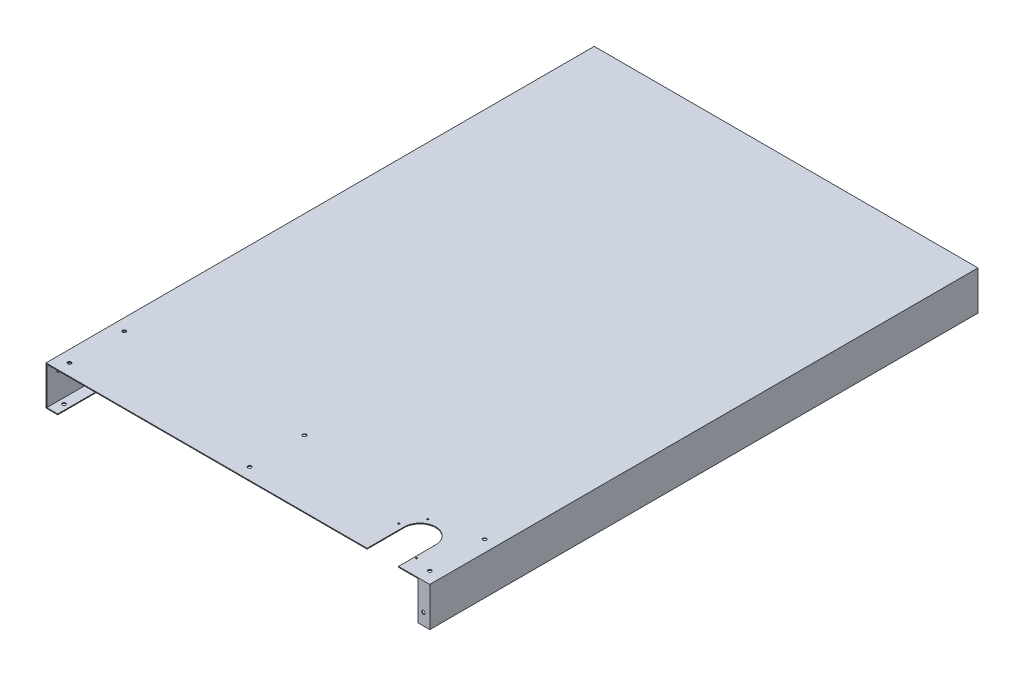
from build123d import *

# Parameters (mm, degrees)
SKETCH_1_W             = 980
SKETCH_1_H             = 1400
EXTRUDE_1_DEPTH        = 100
SHELL_1_T              = -2
CUT_EXTRUDE_1_DEPTH    = 20
SKETCH_5_W             = 976
SKETCH_5_H             = 98
CUT_EXTRUDE_2_DEPTH    = 20
EXTRUDE_2_DEPTH        = 2
SKETCH_7_W             = 2
SKETCH_7_H             = 96
EXTRUDE_3_DEPTH        = 28
SKETCH_8_R             = 4.5
CUT_EXTRUDE_3_DEPTH    = 10
SKETCH_9_R             = 4.5
CUT_EXTRUDE_4_DEPTH    = 10
SKETCH_10_R            = 4.5
CUT_EXTRUDE_5_DEPTH    = 10
SKETCH_11_R            = 4.5
CUT_EXTRUDE_6_DEPTH    = 10
HOLE_WIZARD_M5_1_D     = 4.2
HOLE_WIZARD_M5_1_DEPTH = 1260
HOLE_WIZARD_M5_1_TIP   = 1.2618073


with BuildPart() as part:
    # 草图1 → 凸台-拉伸1 (new body)
    with BuildSketch(Plane(origin=(0, 0, 0), x_dir=(1, 0, 0), z_dir=(0, 1, 0))):
        Rectangle(SKETCH_1_W, SKETCH_1_H)
    extrude(amount=-EXTRUDE_1_DEPTH)

    # 抽壳1
    shell_1_openings = [part.faces().sort_by_distance(p)[0] for p in [
        (0, -100, 0),
    ]]
    offset(amount=SHELL_1_T, openings=shell_1_openings, kind=Kind.INTERSECTION)

    # 草图3 → 切除-拉伸1 (cut)
    with BuildSketch(Plane(origin=(0, 0, 0), x_dir=(1, 0, 0), z_dir=(0, 1, 0))):
        with BuildLine():
            Line((330, -700), (410, -700))
            Line((410, -700), (410, -604.5))
            ThreePointArc((410, -604.5), (370, -564.996875122), (330, -604.5))
            Line((330, -604.5), (330, -700))
        make_face()
    extrude(amount=-CUT_EXTRUDE_1_DEPTH, mode=Mode.SUBTRACT)

    # 草图5 → 切除-拉伸2 (cut)
    with BuildSketch(Plane.XY.offset(700)):
        with Locations((0, -51)):
            Rectangle(SKETCH_5_W, SKETCH_5_H)
    extrude(amount=-CUT_EXTRUDE_2_DEPTH, mode=Mode.SUBTRACT)

    # 草图6 → 凸台-拉伸2 (add)
    with BuildSketch(Plane.XZ.offset(100)):
        Polygon((490, 700), (490, -700), (-490, -700), (-490, 700), (-460, 700), (-460, -670), (460, -670), (460, 700), align=None)
    extrude(amount=-EXTRUDE_2_DEPTH)

    # 草图7 → 凸台-拉伸3 (add)
    with BuildSketch(Plane.ZY.offset(-488)):
        with Locations((699, -50)):
            Rectangle(SKETCH_7_W, SKETCH_7_H)
    extrude(amount=EXTRUDE_3_DEPTH)

    # 草图8 → 切除-拉伸3 (cut)
    with BuildSketch(Plane.XZ.offset(100)):
        with Locations(Location((-474, 670, 0), (0, 0, 270))):
            Circle(SKETCH_8_R)
        with Locations(Location((-474, 0, 0), (0, 0, 270))):
            Circle(SKETCH_8_R)
        with Locations(Location((-474, -684, 0), (0, 0, 270))):
            Circle(SKETCH_8_R)
        with Locations(Location((0, -684, 0), (0, 0, 270))):
            Circle(SKETCH_8_R)
        with Locations(Location((474, -684, 0), (0, 0, 270))):
            Circle(SKETCH_8_R)
        with Locations(Location((474, 0, 0), (0, 0, 270))):
            Circle(SKETCH_8_R)
        with Locations(Location((474, 670, 0), (0, 0, 270))):
            Circle(SKETCH_8_R)
    extrude(amount=-CUT_EXTRUDE_3_DEPTH, mode=Mode.SUBTRACT)

    # 草图9 → 切除-拉伸4 (cut)
    with BuildSketch(Plane(origin=(0, 0, 698), x_dir=(-1, 0, 0), z_dir=(0, 0, -1))):
        with Locations((-474, -70)):
            Circle(SKETCH_9_R)
    extrude(amount=-CUT_EXTRUDE_4_DEPTH, mode=Mode.SUBTRACT)

    # 草图10 → 切除-拉伸5 (cut)
    with BuildSketch(Plane(origin=(-488, 0, 0), x_dir=(0, 0, -1), z_dir=(1, 0, 0))):
        with Locations((-670, -30)):
            Circle(SKETCH_10_R)
        with Locations((-330, -30)):
            Circle(SKETCH_10_R)
    extrude(amount=-CUT_EXTRUDE_5_DEPTH, mode=Mode.SUBTRACT)

    # 草图11 → 切除-拉伸6 (cut)
    with BuildSketch(Plane(origin=(0, 0, 0), x_dir=(1, 0, 0), z_dir=(0, 1, 0))):
        with Locations(Location((-460, -670, 0), (0, 0, 270))):
            Circle(SKETCH_11_R)
        with Locations(Location((0, -530, 0), (0, 0, 270))):
            Circle(SKETCH_11_R)
        with Locations(Location((460, -530, 0), (0, 0, 270))):
            Circle(SKETCH_11_R)
        with Locations(Location((-460, -530, 0), (0, 0, 270))):
            Circle(SKETCH_11_R)
        with Locations(Location((0, -670, 0), (0, 0, 270))):
            Circle(SKETCH_11_R)
        with Locations(Location((460, -670, 0), (0, 0, 270))):
            Circle(SKETCH_11_R)
    extrude(amount=-CUT_EXTRUDE_6_DEPTH, mode=Mode.SUBTRACT)

    # M5 螺纹孔1
    with Locations(Plane(origin=(0, 0, 0), x_dir=(-1, 0, 0), z_dir=(0, 1, 0))):
        with Locations((-343, 558.234628196), (-316, 605), (-415, 659)):
            Hole(HOLE_WIZARD_M5_1_D / 2, depth=HOLE_WIZARD_M5_1_DEPTH)
            with Locations((0, 0, -(HOLE_WIZARD_M5_1_DEPTH + HOLE_WIZARD_M5_1_TIP / 2))):  # 118° drill point
                Cone(0, HOLE_WIZARD_M5_1_D / 2, HOLE_WIZARD_M5_1_TIP, mode=Mode.SUBTRACT)


solid = part.part
